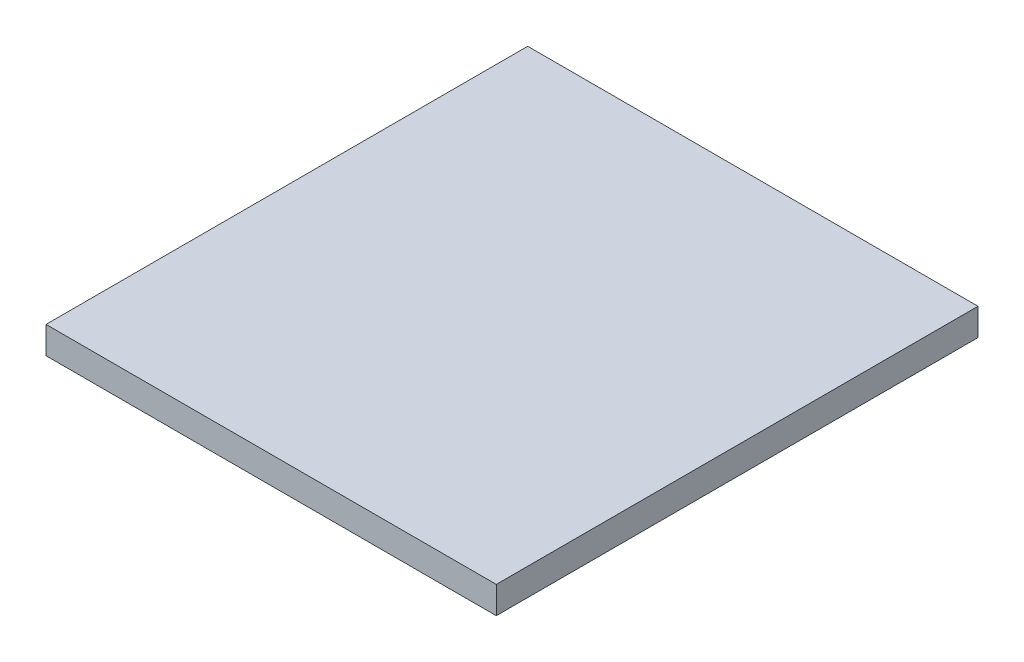
SolidWorks part; units mm, degrees
ref_plane "Front Plane" through (0, 0, 0) normal (0, 0, 1) x (1, 0, 0)
ref_plane "Top Plane" through (0, 0, 0) normal (0, 1, 0) x (1, 0, 0)
ref_plane "Right Plane" through (0, 0, 0) normal (1, 0, 0) x (0, 0, -1)
sketch "Sketch1" plane through (0, 0, 0) normal (0, 1, 0) x (1, 0, 0)
  line L1 (-15.76, -16.86) -> (15.76, -16.86)
  line L2 (-15.76, -16.86) -> (-15.76, 16.86)
  line L3 (-15.76, 16.86) -> (15.76, 16.86)
  line L4 (15.76, -16.86) -> (15.76, 16.86)
  line L5 (-15.76, -16.86) -> (15.76, 16.86) construction
  line L6 (-15.76, 16.86) -> (15.76, -16.86) construction
  point P0 (0, 0)
  dimension "D1" = 31.52
  dimension "D2" = 33.72
extrude "Boss-Extrude1" add sketch "Sketch1" along normal blind 1.9
scale "Scale1" scale about centroid uniform scaling yes scale factor 0.5
